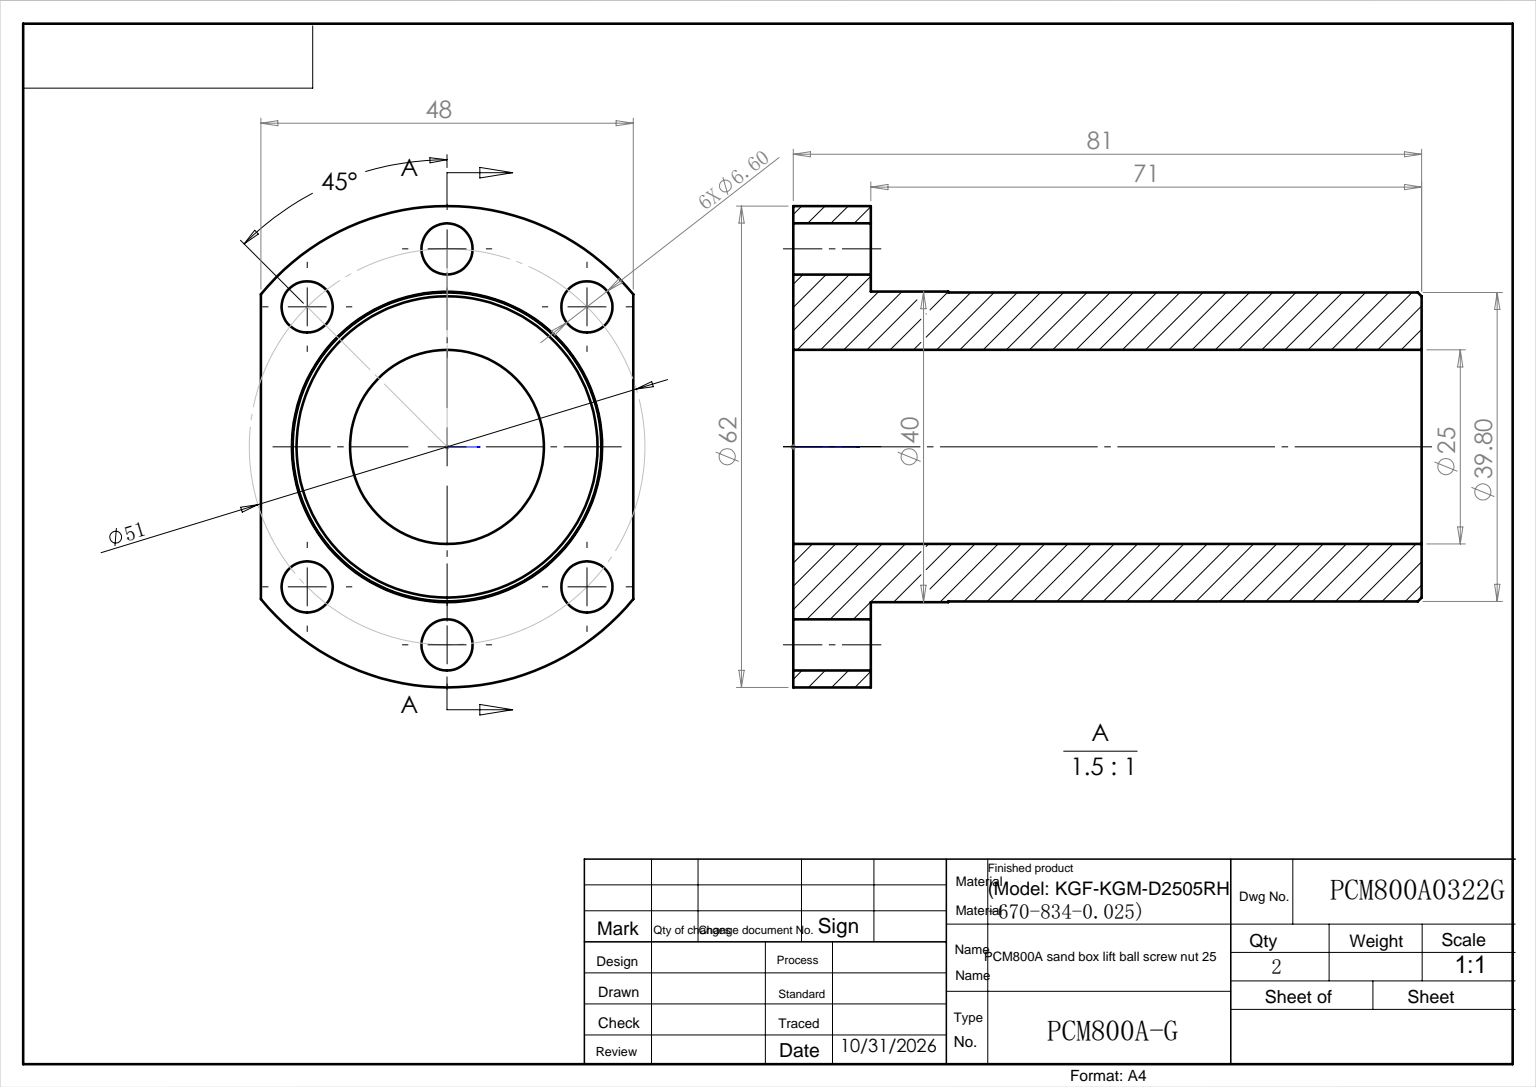
from build123d import *

# Parameters (mm, degrees)
EXTRUDE_1_DEPTH     = 10
SKETCH_2_R          = 20
EXTRUDE_2_DEPTH     = 10
SKETCH_3_R          = 19.9
EXTRUDE_3_DEPTH     = 61
SKETCH_5_R          = 12.5
CUT_EXTRUDE_1_DEPTH = 90.997866916
SKETCH_6_R          = 3.3
CUT_EXTRUDE_2_DEPTH = 90.997866916
CHAMFER_1_SIZE      = 0.5


with BuildPart() as part:
    # 草图1 → 拉伸1 (new body)
    with BuildSketch(Plane(origin=(0, 0, 0), x_dir=(1, 0, 0), z_dir=(0, 1, 0))):
        with BuildLine():
            Line((24, -19.595362506), (24, 19.647471235))
            ThreePointArc((24, 19.647471235), (0, 31.026054364), (-24, 19.647471235))
            Line((-24, 19.647471235), (-24, -19.595362506))
            ThreePointArc((-24, -19.595362506), (0, -30.973945636), (24, -19.595362506))
        make_face()
    extrude(amount=EXTRUDE_1_DEPTH)

    # 草图2 → 拉伸2 (add)
    with BuildSketch(Plane(origin=(0, 10, 0), x_dir=(-1, 0, 0), z_dir=(0, 1, 0))):
        with Locations(Location((0, 0, 0), (0, 0, 90))):
            Circle(SKETCH_2_R)
    extrude(amount=EXTRUDE_2_DEPTH)

    # 草图3 → 拉伸3 (add)
    with BuildSketch(Plane(origin=(0, 20, 0), x_dir=(-1, 0, 0), z_dir=(0, 1, 0))):
        with Locations(Location((0, 0, 0), (0, 0, 270))):
            Circle(SKETCH_3_R)
    extrude(amount=EXTRUDE_3_DEPTH)

    # 草图5 → 切除-拉伸1 (cut, through all)
    with BuildSketch(Plane(origin=(0, 81, 0), x_dir=(-1, 0, 0), z_dir=(0, 1, 0))):
        with Locations(Location((0, 0, 0), (0, 0, 90))):
            Circle(SKETCH_5_R)
    extrude(amount=-CUT_EXTRUDE_1_DEPTH, mode=Mode.SUBTRACT)

    # 草图6 → 切除-拉伸2 (cut, through all)
    with BuildSketch(Plane.XZ):
        with Locations(Location((18.03122292, -18.03122292, 0), (0, 0, 270))):
            Circle(SKETCH_6_R)
        with Locations(Location((0, -25.5, 0), (0, 0, 270))):
            Circle(SKETCH_6_R)
        with Locations(Location((-18.03122292, -18.03122292, 0), (0, 0, 270))):
            Circle(SKETCH_6_R)
        with Locations(Location((-18.03122292, 18.03122292, 0), (0, 0, 270))):
            Circle(SKETCH_6_R)
        with Locations(Location((0, 25.5, 0), (0, 0, 270))):
            Circle(SKETCH_6_R)
        with Locations(Location((18.03122292, 18.03122292, 0), (0, 0, 270))):
            Circle(SKETCH_6_R)
    extrude(amount=-CUT_EXTRUDE_2_DEPTH, mode=Mode.SUBTRACT)

    # 倒角1
    chamfer_1_edges = [part.edges().sort_by_distance(p)[0] for p in [
        (0, 81, 19.9),
    ]]
    chamfer(chamfer_1_edges, length=CHAMFER_1_SIZE)


solid = part.part
